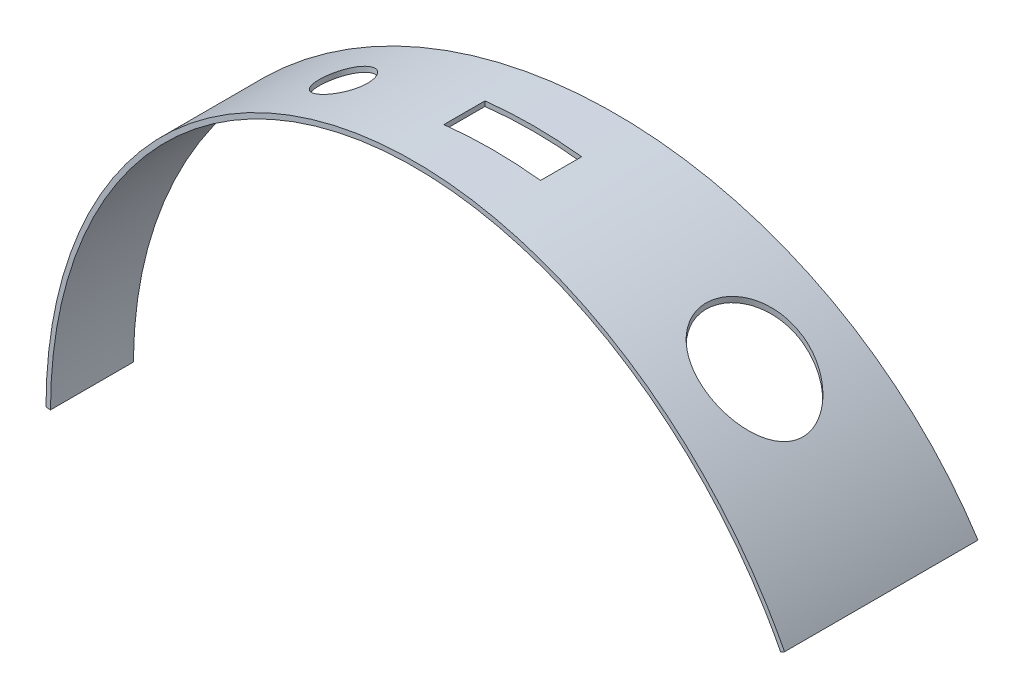
SolidWorks part; units mm, degrees
ref_plane "前视基准面" through (0, 0, 0) normal (0, 0, 1) x (1, 0, 0)
ref_plane "上视基准面" through (0, 0, 0) normal (0, 1, 0) x (1, 0, 0)
ref_plane "右视基准面" through (0, 0, 0) normal (1, 0, 0) x (0, 0, -1)
sketch "草图1" plane through (0, 0, 0) normal (0, 0, 1) x (1, 0, 0)
  line L0 (0, 0) -> (193.865, 111.928) construction
  line L1 (0, 0) -> (-244.5688, 0) construction
  arc A0 (151.5544, 87.5) -> (-175, 0) centre (0, 0) ccw
  dimension "D1" = 175
  dimension "D2" = 30
surface "曲面-拉伸1" sketch "草图1" parameters "D1"=80
thicken "加厚1" surfaces to thicken 106 thickness 1 thickness side both sides parameters "D1"=1
sketch "草图2" plane through (0, 0, 0) normal (0, 1, 0) x (1, 0, 0)
  line L0 (152.4205, 40) -> (-197.5795, 15.5256)
  line L1 (-197.5795, 15.5256) -> (-197.5795, -15.5256)
  line L3 (-197.5795, -15.5256) -> (152.4205, -40)
  line L4 (152.4205, -40) -> (152.4205, 40)
  line L5 (152.4205, 40) -> (-176, 40) construction
  line L6 (-176, -40) -> (152.4205, -40) construction
  dimension "D1" = 4
  dimension "D2" = 4
  dimension "D3" = 350
extrude "切除-拉伸1" cut sketch "草图2" along normal through all flip side to cut
sketch "草图3" plane through (0, 0, 0) normal (0, 1, 0) x (1, 0, 0)
  line L0 (0, 0) -> (0, -74.6276) construction
  line L1 (152.4205, 0) -> (-208.2575, 0) construction
  line L2 (152.4205, 40) -> (152.4205, -40) construction
  line L4 (-20, -8.5) -> (20, -8.5)
  line L5 (-20, -8.5) -> (-20, 8.5)
  line L6 (-20, 8.5) -> (20, 8.5)
  line L7 (20, -8.5) -> (20, 8.5)
  line L8 (-20, -8.5) -> (20, 8.5) construction
  line L9 (-20, 8.5) -> (20, -8.5) construction
  point P7 (0, 0)
  dimension "D1" = 40
  dimension "D2" = 17
extrude "切除-拉伸2" cut sketch "草图3" along normal up to surface (174.8599 mm away)
sketch "草图4" plane through (0, 0, 0) normal (0, 1, 0) x (1, 0, 0)
  line L0 (152.4205, 0) -> (-216.0243, 0) construction
  line L1 (152.4205, 40) -> (152.4205, -40) construction
  circle A0 centre (100, 0) radius 20
  dimension "D1" = 40
  dimension "D2" = 100
extrude "切除-拉伸3" cut sketch "草图4" along normal up to surface (144.8309 mm away)
sketch "草图5" plane through (0, 0, 0) normal (0, 1, 0) x (1, 0, 0)
  line L0 (152.4205, 0) -> (-176, 0) construction
  line L1 (152.4205, 40) -> (152.4205, -40) construction
  line L2 (-176, 17.0346) -> (-176, -17.0346) construction
  circle A0 centre (-70, 0) radius 10
  dimension "D1" = 20
  dimension "D2" = 70
extrude "切除-拉伸4" cut sketch "草图5" along normal up to surface (161.4806 mm away)
